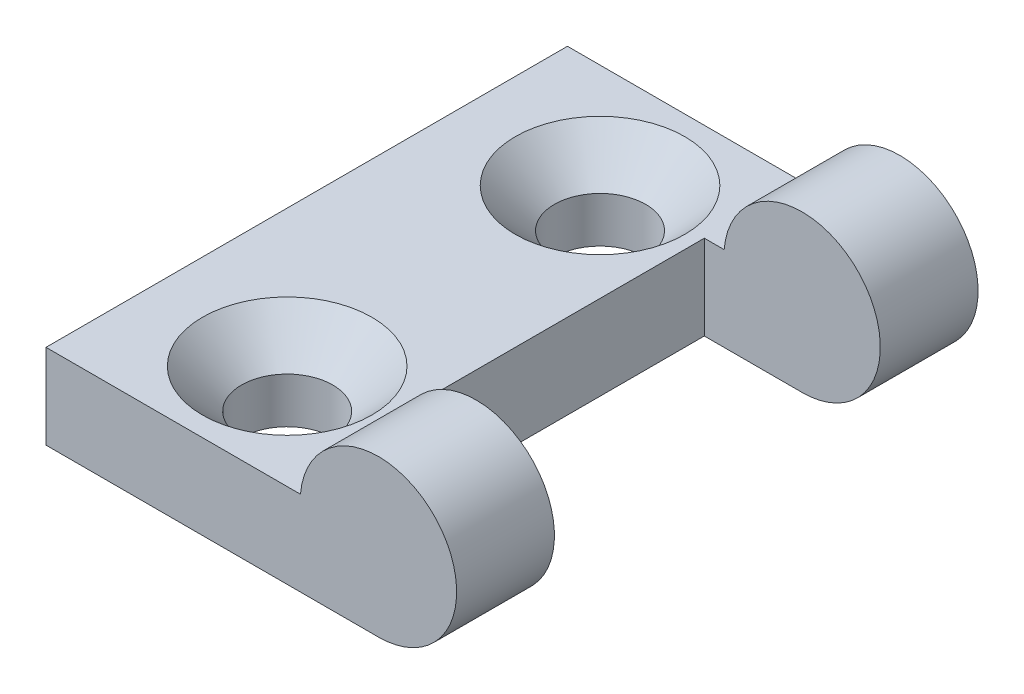
from build123d import *

# Parameters (mm, degrees)
SKETCH_1_W          = 25.5
SKETCH_1_H          = 40
EXTRUDE_1_DEPTH     = 6.5
SKETCH_2_R          = 6
EXTRUDE_2_DEPTH     = 40
SKETCH_3_W          = 27
SKETCH_3_H          = 25
CUT_EXTRUDE_1_DEPTH = 30.925950277
SKETCH_5_R          = 3.5
CUT_EXTRUDE_2_DEPTH = 29.174678348
CHAMFER_1_SIZE      = 3


with BuildPart() as part:
    # 草图1 → 凸台-拉伸1 (new body)
    with BuildSketch(Plane(origin=(0, 0, 0), x_dir=(1, 0, 0), z_dir=(0, 1, 0))):
        Rectangle(SKETCH_1_W, SKETCH_1_H)
    extrude(amount=EXTRUDE_1_DEPTH)

    # 草图2 → 凸台-拉伸2 (add)
    with BuildSketch(Plane.XY.offset(20)):
        with Locations((12.75, 6)):
            Circle(SKETCH_2_R)
    extrude(amount=-EXTRUDE_2_DEPTH)

    # 草图3 → 切除-拉伸1 (cut, through all)
    with BuildSketch(Plane.XZ):
        with Locations((18.75, 0)):
            Rectangle(SKETCH_3_W, SKETCH_3_H)
    extrude(amount=-CUT_EXTRUDE_1_DEPTH, mode=Mode.SUBTRACT)

    # 草图5 → 切除-拉伸2 (cut, through all)
    with BuildSketch(Plane(origin=(0, 6.5, 0), x_dir=(1, 0, 0), z_dir=(0, 1, 0))):
        with Locations(Location((-2.25, 12, 0), (0, 0, 270))):
            Circle(SKETCH_5_R)
        with Locations(Location((-2.25, -12, 0), (0, 0, 270))):
            Circle(SKETCH_5_R)
    extrude(amount=-CUT_EXTRUDE_2_DEPTH, mode=Mode.SUBTRACT)

    # 倒角1
    chamfer_1_edges = [part.edges().sort_by_distance(p)[0] for p in [
        (-2.25, 6.5, -15.5),
        (-2.25, 6.5, 8.5),
    ]]
    chamfer(chamfer_1_edges, length=CHAMFER_1_SIZE)


solid = part.part
